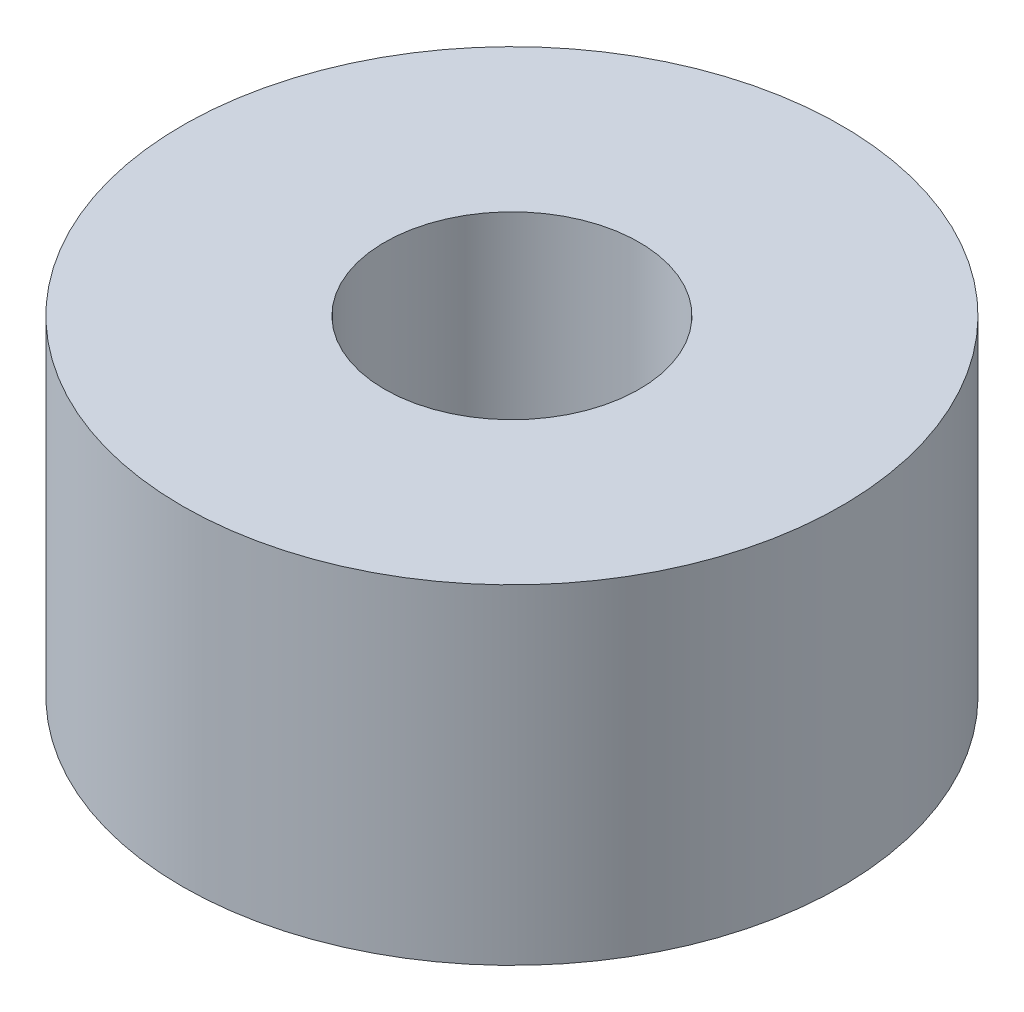
SolidWorks part; units mm, degrees
material "SS400B"
ref_plane "Front Plane" through (0, 0, 0) normal (0, 0, 1) x (1, 0, 0)
ref_plane "Top Plane" through (0, 0, 0) normal (0, 1, 0) x (1, 0, 0)
ref_plane "Right Plane" through (0, 0, 0) normal (1, 0, 0) x (0, 0, -1)
sketch "Sketch1" plane through (0, 0, 0) normal (0, 1, 0) x (1, 0, 0)
  circle A0 centre (0, 0) radius 11
  circle A1 centre (0, 0) radius 4
  dimension "D1" = 22
  dimension "D2" = 8
extrude "Boss-Extrude1" add sketch "Sketch1" along normal blind 11
hole_wizard "M10 Tapped Hole1" positions "Sketch2" profile "Sketch3" tap size "M10" standard "GB"
sketch "Sketch2" plane through (0, 11, 0) normal (0, 1, 0) x (1, 0, 0)
  point P0 (0, 0)
sketch "Sketch3" plane through (0, 11, 0) normal (1, 0, 0) x (0, 0, 1)
  line L0 (0, 0) -> (0, 27.0537)
  line L1 (0, 27.0537) -> (4.25, 24.5)
  line L2 (4.25, 24.5) -> (4.25, 0)
  line L5 (4.25, 0) -> (0, 0)
  line L10 (0, 27.0537) -> (-4.25, 24.5) construction
  line L11 (0, -6.35) -> (0, 107.95) construction
  dimension "螺纹孔钻头直径" = 8.5
  dimension "螺纹孔钻头深度" = 24.5
  dimension "导头角度" = 118
cosmetic thread "Cosmetic Thread1" parameters "D1"=20, "D2"=10
